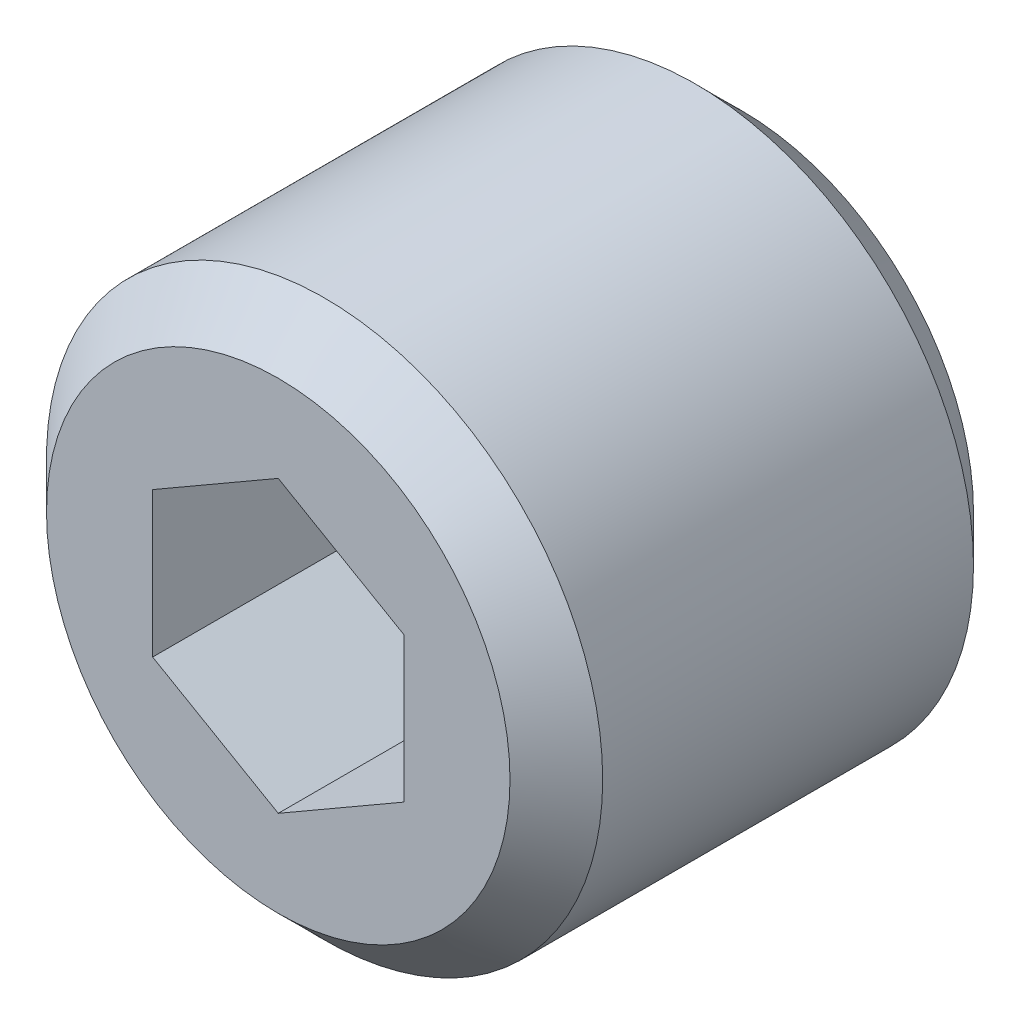
from build123d import *

# Parameters (mm, degrees)
SKETCH1_R           = 6
BOSS_EXTRUDE1_DEPTH = 10
CUT_EXTRUDE1_DEPTH  = 5
CHAMFER1_SIZE       = 1


with BuildPart() as part:
    # Sketch1 → Boss-Extrude1 (new body)
    with BuildSketch(Plane.XY):
        Circle(SKETCH1_R)
    extrude(amount=BOSS_EXTRUDE1_DEPTH)

    # Sketch2 → Cut-Extrude1 (cut)
    with BuildSketch(Plane.XY.offset(10)):
        Polygon((0, 3.129298789), (-2.710052247, 1.564649395), (-2.710052247, -1.564649395), (0, -3.129298789), (2.710052247, -1.564649395), (2.710052247, 1.564649395), align=None)
    extrude(amount=-CUT_EXTRUDE1_DEPTH, mode=Mode.SUBTRACT)

    # Chamfer1
    chamfer1_edges = [part.edges().sort_by_distance(p)[0] for p in [
        (-6, 0, 0),
        (-6, 0, 10),
    ]]
    chamfer(chamfer1_edges, length=CHAMFER1_SIZE)


solid = part.part
